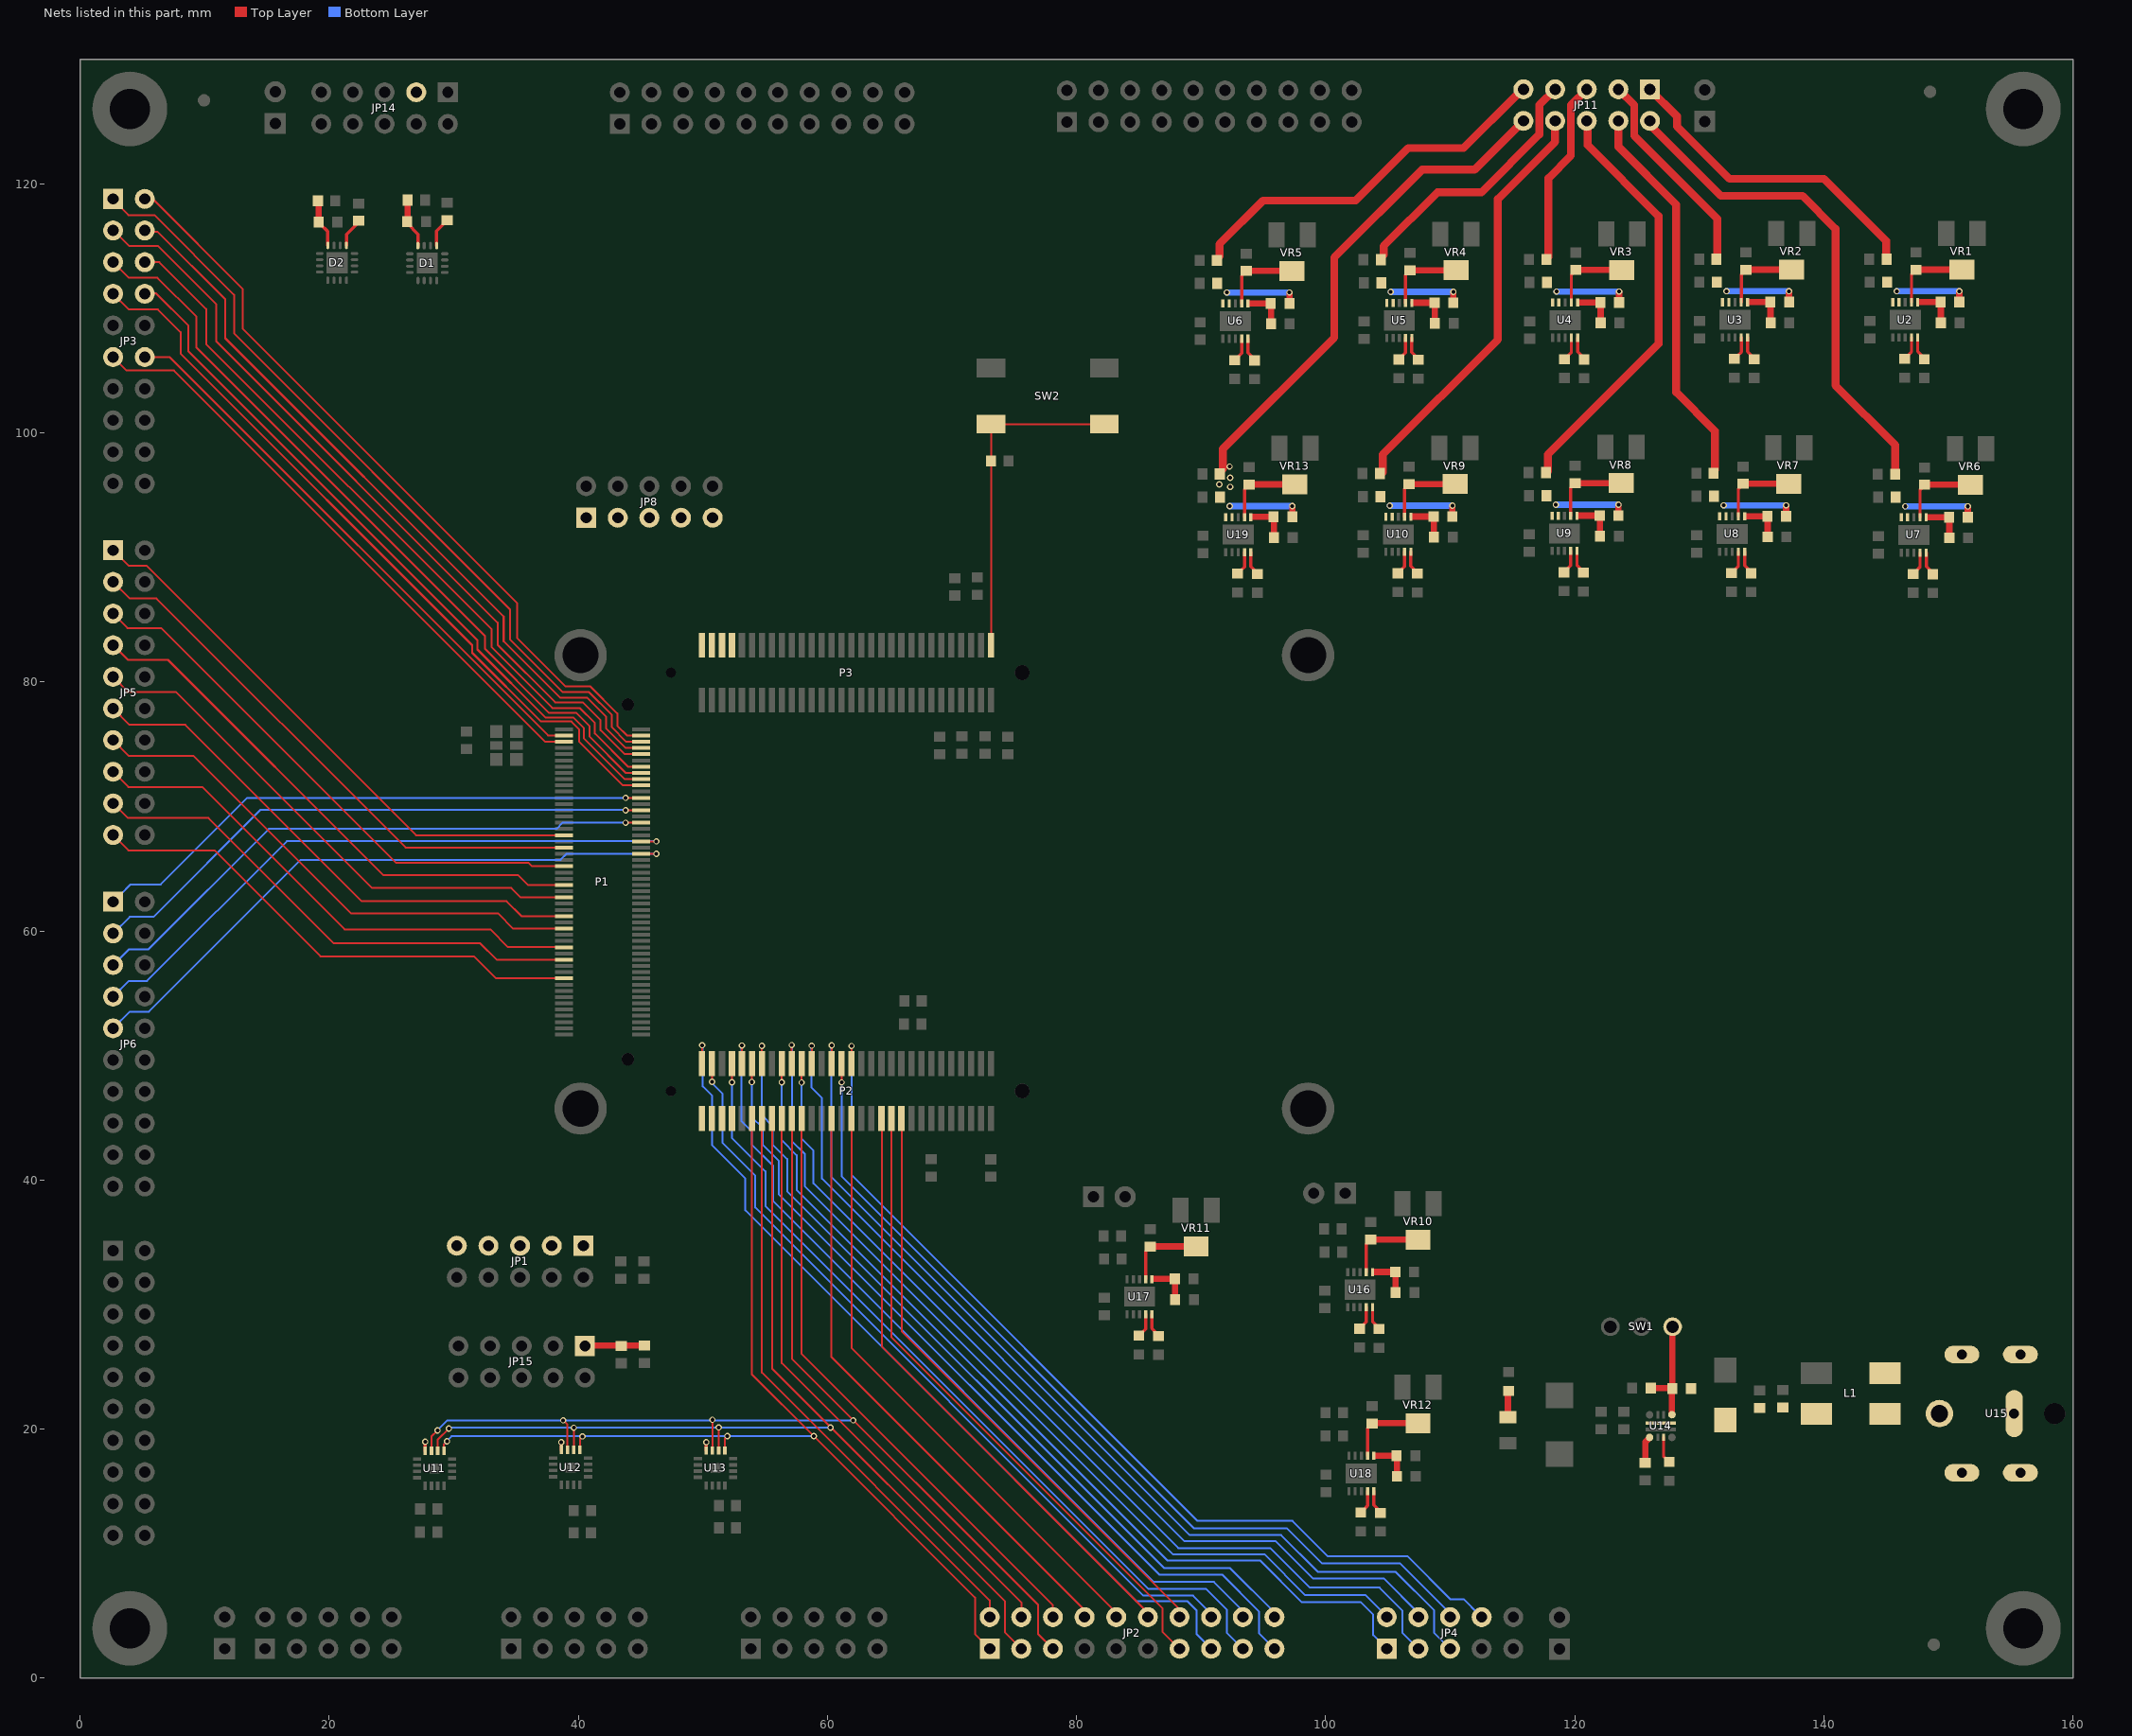
[diagram p0: the nets of this part, all layers, seen from the top]
# Altium PCB MISC82195.PcbDoc (part 5 of 8)
Units mm, origin at the board's own origin, x right, y up, seen from the top; angles counter-clockwise.
Board outline 160 x 130 mm, 4 copper layers (Top Layer, GND, POWER, Bottom Layer); 214 components, 251 nets, 1068 pads, 1218 vias.

## Via types
v1: diameter 0.508, hole 0.305, Top Layer to Bottom Layer, 1218 vias

## Nets (pads, with @x,y where several pads share a name; then routed paths per layer and width w, separated by ;. In a path a pad name is that pad's centre, name@x,y a point inside that pad or via, vN(x,y) a via of type N, cw(c..) or ccw(c..) an arc to the next point about the centre after c; other vN are vias at no path point) (continued)
LDO_1: C14.2 C15.2 JP11.1 R1.2 U2.9 U2.10 | length 31.8
  Top Layer w0.508: R1.2@150.86,110.49 v1(150.86,111.363)
  Top Layer w0.635: JP11.1@126.035,127.584 128.194,125.425 128.194,124.612 132.41,120.396 140.005,120.396 144.983,115.418 C14.2@144.983,113.995
  Bottom Layer w0.508: v1(145.838,111.363) v1(150.86,111.363)
LDO_2: C17.2 C18.2 JP11.3 R2.2 U3.9 U3.10 | length 22.5
  Top Layer w0.508: R2.2@137.194,110.49 v1(137.194,111.363)
  Top Layer w0.635: JP11.3@123.495,127.584 124.765,126.314 124.765,123.85 131.445,117.17 C17.2@131.445,114.3
  Bottom Layer w0.508: v1(132.173,111.363) v1(137.194,111.363)
LDO_3: C20.2 C21.2 JP11.5 R3.2 U4.9 U4.10 | length 20.6
  Top Layer w0.508: R3.2@123.555,110.465 v1(123.555,111.337)
  Top Layer w0.635: C20.2@117.881,114.122 117.881,120.447 119.685,122.25 119.685,126.314 JP11.5@120.955,127.584
  Bottom Layer w0.508: v1(118.533,111.337) v1(123.555,111.337)
LDO_4: C26.2 C27.2 JP11.7 R13.2 U5.9 U5.10 | length 26.9
  Top Layer w0.508: R13.2@110.245,110.439 v1(110.245,111.312)
  Top Layer w0.635: C26.2@104.648,114.3 104.648,114.986 108.966,119.304 112.497,119.304 117.145,123.952 117.145,126.314 JP11.7@118.415,127.584
  Bottom Layer w0.508: v1(105.223,111.312) v1(110.245,111.312)
LDO_5: C29.2 C30.2 JP11.9 R14.2 U6.9 U6.10 | length 36.4
  Top Layer w0.508: R14.2@97.088,110.388 v1(97.088,111.261)
  Top Layer w0.635: C29.2@91.465,114.173 91.465,115.138 94.971,118.643 102.413,118.643 106.629,122.86 111.074,122.86 JP11.9@115.443,127.229 ; JP11.9@115.494,127.178 JP11.9@115.545,127.229 ; JP11.9@115.532,127.241 JP11.9@115.875,127.584
  Bottom Layer w0.508: v1(92.066,111.261) v1(97.088,111.261)
LDO_6: C32.2 C33.2 JP11.2 R15.2 U7.9 U7.10 | length 46.2
  Top Layer w0.508: R15.2@151.545,93.218 v1(151.545,94.091)
  Top Layer w0.635: JP11.2@126.035,125.044 126.035,124.714 131.724,119.024 138.278,119.024 140.919,116.383 140.919,103.81 145.72,99.009 C32.2@145.72,96.774
  Bottom Layer w0.508: v1(146.524,94.091) v1(151.545,94.091)
LDO_7: C38.2 C39.2 JP11.4 R25.2 U8.9 U8.10 | length 37.1
  Top Layer w0.508: R25.2@136.966,93.294 v1(136.966,94.167)
  Top Layer w0.635: JP11.4@123.495,125.044 123.495,122.961 128.143,118.313 128.143,103.251 131.242,100.152 C38.2@131.242,97.028
  Bottom Layer w0.508: v1(131.944,94.167) v1(136.966,94.167)
LDO_8: C41.2 C42.2 JP11.6 R26.2 U9.9 U9.10 | length 40.1
  Top Layer w0.508: R26.2@123.504,93.345 v1(123.504,94.218)
  Top Layer w0.635: C41.2@117.831,96.901 117.831,98.247 126.721,107.137 126.721,117.399 121.031,123.088 JP11.6@121.031,124.892 ; JP11.6@120.955,124.892 JP11.6@120.955,125.044
  Bottom Layer w0.508: v1(118.482,94.218) v1(123.504,94.218)
LDO_9: C44.2 C45.2 JP11.8 R27.2 U10.9 U10.10 | length 39.8
  Top Layer w0.508: R27.2@110.169,93.269 v1(110.169,94.141)
  Top Layer w0.635: C44.2@104.572,96.825 104.572,98.247 113.817,107.493 113.817,118.77 118.415,123.368 JP11.8@118.415,125.044
  Bottom Layer w0.508: v1(105.147,94.141) v1(110.169,94.141)
LDO_10: C81.2 C82.2 JP11.10 JP14.3 R55.2 U11.16 U12.16 U13.16 U19.9 U19.10 | length 48.3
  Top Layer w0.279: U11.16@27.714,18.258 v1(27.714,18.977) ; v1(38.633,18.948) 38.636,18.946 U12.16@38.636,18.334 ; U13.16@50.269,18.283 v1(50.269,18.946)
  Top Layer w0.508: R55.2@97.316,93.243 v1(97.316,94.116)
  Top Layer w0.635: C81.2@91.745,97.104 91.745,98.704 100.686,107.645 100.686,114.071 107.747,121.133 111.963,121.133 JP11.10@115.875,125.044
  Bottom Layer w0.508: v1(92.295,94.116) v1(97.316,94.116)
  other v1: 92.329,95.656 91.465,95.86 92.329,96.393 92.278,97.282
M_RESET_IN_N: C8.1 P3.C59 SW2.3 SW2.4 | length 26.4
  Top Layer w0.152: SW2.3@73.123,100.696 SW2.4@81.9,100.696 ; P3.C59@73.137,82.939 73.137,99.212 SW2.3@73.137,100.573
NetC22_2: C22.2 U2.7 VR1.2 | length 6.4
  Top Layer w0.254: U2.7@147.025,110.479 147.025,112.71 C22.2@147.295,112.979
  Top Layer w0.508: C22.2@147.292,113.104 VR1.2@151.071,113.104
NetC23_2: C23.2 U3.7 VR2.2 | length 6.4
  Top Layer w0.254: U3.7@133.36,110.479 133.36,112.71 C23.2@133.629,112.979
  Top Layer w0.508: C23.2@133.627,113.104 VR2.2@137.406,113.104
NetC24_2: C24.2 U4.7 VR3.2 | length 6.4
  Top Layer w0.254: U4.7@119.72,110.454 119.72,112.684 C24.2@119.99,112.954
  Top Layer w0.508: C24.2@119.987,113.079 VR3.2@123.766,113.079
NetC34_2: C34.2 U5.7 VR4.2 | length 6.4
  Top Layer w0.254: U5.7@106.41,110.428 106.41,112.659 C34.2@106.68,112.928
  Top Layer w0.508: C34.2@106.678,113.053 VR4.2@110.457,113.053
NetC35_2: C35.2 U6.7 VR5.2 | length 6.4
  Top Layer w0.254: U6.7@93.253,110.377 93.253,112.608 C35.2@93.523,112.878
  Top Layer w0.508: C35.2@93.521,113.002 VR5.2@97.3,113.002
NetC36_2: C36.2 U7.7 VR6.2 | length 6.4
  Top Layer w0.254: U7.7@147.711,93.207 147.711,95.438 C36.2@147.98,95.707
  Top Layer w0.508: C36.2@147.978,95.832 VR6.2@151.757,95.832
NetC46_2: C46.2 U8.7 VR7.2 | length 6.4
  Top Layer w0.254: U8.7@133.131,93.283 133.131,95.514 C46.2@133.401,95.783
  Top Layer w0.508: C46.2@133.399,95.908 VR7.2@137.178,95.908
NetC47_2: C47.2 U9.7 VR8.2 | length 6.4
  Top Layer w0.254: U9.7@119.669,93.334 119.669,95.565 C47.2@119.939,95.834
  Top Layer w0.508: C47.2@119.937,95.959 VR8.2@123.716,95.959
NetC48_2: C48.2 U10.7 VR9.2 | length 6.4
  Top Layer w0.254: U10.7@106.334,93.258 106.334,95.488 C48.2@106.604,95.758
  Top Layer w0.508: C48.2@106.602,95.883 VR9.2@110.381,95.883
NetC57_2: C57.2 D1.16 R37.1 | length 4
  Top Layer w0.254: R37.1@26.289,117.016 26.289,116.789 27.13,115.948 D1.16@27.13,115.024
  Top Layer w0.508: R37.1@26.291,117.016 C57.2@26.291,118.679
NetC58_1: C58.1 D1.13 | length 2.1
  Top Layer w0.254: D1.13@28.63,115.024 28.63,116.209 C58.1@29.286,116.865
NetC59_2: C59.2 D2.16 R38.1 | length 3.6
  Top Layer w0.254: R38.1@19.329,116.738 19.891,116.177 D2.16@19.891,115.05
  Top Layer w0.508: R38.1@19.151,116.926 C59.2@19.151,118.592
NetC60_1: C60.1 D2.13 | length 2.2
  Top Layer w0.254: D2.13@21.391,115.05 21.391,115.93 C60.1@22.301,116.84
NetC61_2: C61.2 C62.2 JP15.1 | length 4.6
  Top Layer w0.508: JP15.1@40.752,26.711 C62.2@45.323,26.711
NetC65_2: C65.2 C66.2 D4.2 L1.4 R41.1 U14.5
NetC67_2: C67.2 U14.7 | length 2.2
  Top Layer w0.508: C67.2@125.774,17.406 C67.2@125.654,17.286 125.654,18.948 U14.7@125.882,19.177
NetC77_2: C77.2 U16.7 VR10.2 | length 6.9
  Top Layer w0.254: U16.7@103.261,32.603 103.261,34.833 C77.2@103.53,35.103
  Top Layer w0.508: C77.2@103.528,35.228 107.417,35.228 107.698,35.228 VR10.2@107.747,35.179
NetC78_2: C78.2 U17.7 VR11.2 | length 6.4
  Top Layer w0.254: U17.7@85.557,32.044 85.557,34.274 C78.2@85.827,34.544
  Top Layer w0.508: C78.2@85.824,34.669 VR11.2@89.603,34.669
NetC79_2: C79.2 U18.7 VR12.2 | length 6.4
  Top Layer w0.254: U18.7@103.362,17.845 103.362,20.076 C79.2@103.632,20.345
  Top Layer w0.508: C79.2@103.63,20.47 VR12.2@107.409,20.47
NetC83_2: C83.2 U19.7 VR13.2 | length 6.4
  Top Layer w0.254: U19.7@93.482,93.232 93.482,95.463 C83.2@93.751,95.733
  Top Layer w0.508: C83.2@93.749,95.857 VR13.2@97.528,95.857
NetJP1_1: JP1.1 JP1.3 JP1.5 JP1.7 JP1.9 P2.A2 P2.A4 P2.A6 P2.A8
NetJP8_1: JP8.1 JP8.3 JP8.5 JP8.7 JP8.9 P3.C1 P3.C3 P3.C5 P3.C7
NetL1_1: L1.1 U15.1
NetL1_2: L1.2 U15.2 U15.3
NetLED1_2: LED1.2 R42.2 | length 1.9
  Top Layer w0.508: LED1.2@114.63,20.964 R42.2@114.63,22.835
NetR1_1: R1.1 R7.2 U2.6 | length 3.4
  Top Layer w0.508: 147.676,110.491 149.378,110.491 R7.2@149.378,108.839
NetR2_1: R2.1 R8.2 U3.6 | length 3.4
  Top Layer w0.508: 134.011,110.491 135.713,110.491 R8.2@135.713,108.839
NetR3_1: R3.1 R9.2 U4.6 | length 3.4
  Top Layer w0.508: 120.371,110.465 122.073,110.465 R9.2@122.073,108.814
NetR4_1: R4.1 U2.4 | length 1.6
  Top Layer w0.254: R4.1@146.71,106.172 147.025,106.487 U2.4@147.025,107.656
NetR5_1: R5.1 U3.4 | length 1.6
  Top Layer w0.254: R5.1@133.045,106.172 133.36,106.487 U3.4@133.36,107.656
NetR6_1: R6.1 U4.4 | length 1.6
  Top Layer w0.254: R6.1@119.405,106.147 119.72,106.461 U4.4@119.72,107.631
NetR10_2: R10.2 U2.5 | length 1.7
  Top Layer w0.254: U2.5@147.525,107.656 147.525,106.526 R10.2@147.904,106.147
NetR11_2: R11.2 U3.5 | length 1.7
  Top Layer w0.254: U3.5@133.86,107.656 133.86,106.526 R11.2@134.239,106.147
NetR12_2: R12.2 U4.5 | length 1.7
  Top Layer w0.254: U4.5@120.22,107.631 120.22,106.501 R12.2@120.599,106.121
NetR13_1: R13.1 R19.2 U5.6 | length 3.4
  Top Layer w0.508: 107.062,110.44 108.764,110.44 R19.2@108.764,108.788
NetR14_1: R14.1 R20.2 U6.6 | length 3.4
  Top Layer w0.508: 93.905,110.389 95.606,110.389 R20.2@95.606,108.737
NetR15_1: R15.1 R21.2 U7.6 | length 3.4
  Top Layer w0.508: 148.362,93.219 150.064,93.219 R21.2@150.064,91.567
NetR16_1: R16.1 U5.4 | length 1.6
  Top Layer w0.254: R16.1@106.096,106.121 106.41,106.436 U5.4@106.41,107.605
NetR17_1: R17.1 U6.4 | length 1.6
  Top Layer w0.254: R17.1@92.939,106.07 93.253,106.385 U6.4@93.253,107.555
NetR18_1: R18.1 U7.4 | length 1.6
  Top Layer w0.254: R18.1@147.396,88.9 147.711,89.215 U7.4@147.711,90.384
NetR22_2: R22.2 U5.5 | length 1.7
  Top Layer w0.254: U5.5@106.91,107.605 106.91,106.475 R22.2@107.29,106.096
NetR23_2: R23.2 U6.5 | length 1.7
  Top Layer w0.254: U6.5@93.753,107.555 93.753,106.424 R23.2@94.132,106.045
NetR24_2: R24.2 U7.5 | length 1.7
  Top Layer w0.254: U7.5@148.211,90.384 148.211,89.254 R24.2@148.59,88.875
NetR25_1: R25.1 R31.2 U8.6 | length 3.4
  Top Layer w0.508: 133.783,93.295 135.484,93.295 R31.2@135.484,91.643
NetR26_1: R26.1 R32.2 U9.6 | length 3.4
  Top Layer w0.508: 120.321,93.346 122.022,93.346 R32.2@122.022,91.694
NetR27_1: R27.1 R33.2 U10.6 | length 3.4
  Top Layer w0.508: 106.986,93.27 108.687,93.27 R33.2@108.687,91.618
NetR28_1: R28.1 U8.4 | length 1.6
  Top Layer w0.254: R28.1@132.817,88.976 133.131,89.291 U8.4@133.131,90.46
NetR29_1: R29.1 U9.4 | length 1.6
  Top Layer w0.254: R29.1@119.355,89.027 119.669,89.342 U9.4@119.669,90.511
NetR30_1: R30.1 U10.4 | length 1.6
  Top Layer w0.254: R30.1@106.02,88.951 106.334,89.265 U10.4@106.334,90.435
NetR34_2: R34.2 U8.5 | length 1.7
  Top Layer w0.254: U8.5@133.631,90.46 133.631,89.33 R34.2@134.01,88.951
NetR35_2: R35.2 U9.5 | length 1.7
  Top Layer w0.254: U9.5@120.169,90.511 120.169,89.381 R35.2@120.548,89.002
NetR36_2: R36.2 U10.5 | length 1.7
  Top Layer w0.254: U10.5@106.834,90.435 106.834,89.305 R36.2@107.213,88.925
NetR39_1: R39.1 R41.2 SW1.3 U14.1 | length 8.7
  Top Layer w0.508: R39.1@126.213,23.292 127.787,23.292 127.798,23.281 U14.1@127.798,21.159 ; R41.2@127.821,23.266 SW1.3@127.821,28.253
NetR40_1: R40.1 U14.9 | length 1.9
  Top Layer w0.254: U14.9@127.123,19.339 127.123,17.834 R40.1@127.381,17.577
NetR43_1: R43.1 R49.2 U16.6 | length 3.4
  Top Layer w0.508: 103.912,32.614 105.614,32.614 R49.2@105.614,30.963
NetR44_1: R44.1 R50.2 U17.6 | length 3.4
  Top Layer w0.508: 86.208,32.056 87.91,32.056 R50.2@87.91,30.404
NetR45_1: R45.1 R51.2 U18.6 | length 3.4
  Top Layer w0.508: 104.014,17.857 105.716,17.857 R51.2@105.716,16.205
NetR46_1: R46.1 U16.4 | length 1.6
  Top Layer w0.254: R46.1@102.946,28.296 103.261,28.61 U16.4@103.261,29.78
NetR47_1: R47.1 U17.4 | length 1.6
  Top Layer w0.254: R47.1@85.242,27.737 85.557,28.051 U17.4@85.557,29.221
NetR48_1: R48.1 U18.4 | length 1.6
  Top Layer w0.254: R48.1@103.048,13.538 103.362,13.853 U18.4@103.362,15.022
NetR52_2: R52.2 U16.5 | length 1.7
  Top Layer w0.254: U16.5@103.761,29.78 103.761,28.65 R52.2@104.14,28.27
NetR53_2: R53.2 U17.5 | length 1.7
  Top Layer w0.254: U17.5@86.057,29.221 86.057,28.091 R53.2@86.436,27.711
NetR54_2: R54.2 U18.5 | length 1.7
  Top Layer w0.254: U18.5@103.862,15.022 103.862,13.892 R54.2@104.242,13.513
NetR55_1: R55.1 R57.2 U19.6 | length 3.4
  Top Layer w0.508: 94.133,93.244 95.835,93.244 R57.2@95.835,91.592
NetR56_1: R56.1 U19.4 | length 1.6
  Top Layer w0.254: R56.1@93.167,88.925 93.482,89.24 U19.4@93.482,90.41
NetR58_2: R58.2 U19.5 | length 1.7
  Top Layer w0.254: U19.5@93.982,90.41 93.982,89.279 R58.2@94.361,88.9
PW1: JP2.1 P2.A12 U11.13 U12.13 U13.13 | length 83.7
  Top Layer w0.152: U11.13@29.214,18.258 29.214,18.775 v1(29.464,19.025) ; U12.13@40.136,18.334 40.136,19.207 v1(40.335,19.406) ; U13.13@51.769,18.521 U13.13@51.769,18.283 51.769,19.232 v1(51.968,19.431) ; P2.A12@53.937,44.938 53.924,44.925 53.924,24.409 v1@58.877,19.456 ; v1(58.903,19.431) v1@58.877,19.456 ; JP2.1@73.025,2.362 71.857,3.531 71.857,6.477 v1@58.877,19.456
  Bottom Layer w0.152: v1@29.515,19.126 29.82,19.431 30.353,19.431 ; 30.15,19.431 30.353,19.431 ; v1@58.877,19.431 v1(51.968,19.431) 30.353,19.431
PW2: JP2.3 P2.A16 U11.14 U12.14 U13.14 | length 87.3
  Top Layer w0.152: U11.14@28.714,18.258 28.714,19.138 v1(29.616,20.041) ; U12.14@39.636,18.334 v1(39.636,20.105) ; U13.14@51.269,18.283 v1(51.269,20.129) ; P2.A16@55.55,44.926 55.55,24.867 74.27,6.147 74.27,3.658 JP2.3@75.565,2.362
  Bottom Layer w0.152: v1@29.667,20.117 60.274,20.117 v1(60.249,20.117)
PW3: JP2.5 P2.A20 U11.15 U12.15 U13.15 | length 91.6
  Top Layer w0.152: U11.15@28.214,18.258 28.214,19.4 v1(28.702,19.888) ; v1(38.786,20.701) 39.136,20.351 U12.15@39.136,18.334 ; U13.15@50.769,18.283 v1(50.769,20.747) ; P2.A20@57.15,44.926 57.15,25.654 76.911,5.893 76.911,3.556 JP2.5@78.105,2.362
  Bottom Layer w0.152: v1@28.804,20.015 29.489,20.701 v1(38.786,20.701) v1(62.078,20.701)
PW7: JP2.13 P2.A40 | length 52.1
  Top Layer w0.152: P2.A40@65.151,44.925 65.151,27.356 86.919,5.588 86.919,3.708 JP2.13@88.265,2.362
PW8: JP2.15 P2.A1 | length 69.5
  Top Layer w0.152: P2.A1@49.937,49.338 v1(49.937,50.824)
  Bottom Layer w0.152: v1@49.987,50.749 49.987,47.523 50.724,46.787 50.724,46.38 ; 50.724,46.685 50.724,46.38 ; JP2.15@90.805,2.362 89.637,3.531 89.637,5.436 88.875,6.198 84.785,6.198 53.416,37.567 53.416,40.107 50.724,42.799 50.724,46.38
PW9: JP2.17 P2.A7 | length 66.7
  Top Layer w0.152: v1(52.337,47.842) P2.A7@52.337,49.338
  Bottom Layer w0.152: v1@52.451,47.828 52.324,47.701 52.324,43.383 55.016,40.691 55.016,37.922 85.776,7.163 90.399,7.163 92.075,5.486 92.075,3.632 JP2.17@93.345,2.362
PW10: JP2.19 P2.A11 | length 67.3
  Top Layer w0.152: v1(53.937,47.866) P2.A11@53.937,49.338
  Bottom Layer w0.152: v1@53.924,47.828 53.924,45.06 54.813,44.171 54.813,42.824 56.109,41.529 56.109,38.837 86.639,8.306 91.694,8.306 94.64,5.359 94.64,3.607 JP2.19@95.885,2.362
PW11: JP4.1 P2.A17 | length 74.3
  Top Layer w0.152: v1(56.337,47.854) P2.A17@56.337,49.338
  Bottom Layer w0.152: v1@56.337,47.955 56.337,43.18 57.531,41.986 57.531,39.218 87.3,9.449 94.742,9.449 98.095,6.096 102.819,6.096 103.81,5.105 103.81,3.454 JP4.1@104.902,2.362
PW12: JP4.3 P2.A21 | length 75.1
  Top Layer w0.152: v1(57.937,47.828) P2.A21@57.937,49.338
  Bottom Layer w0.152: v1@58.014,47.854 57.937,47.777 57.937,43.307 58.877,42.367 58.877,39.726 88.163,10.439 95.555,10.439 98.73,7.264 104.318,7.264 106.172,5.41 106.172,3.632 JP4.3@107.442,2.362
PW13: JP4.5 P2.A27 | length 78.4
  Top Layer w0.152: P2.A27@60.337,49.338 v1(60.337,50.812)
  Bottom Layer w0.152: v1@60.325,50.724 60.325,40.234 89.078,11.481 96.418,11.481 99.365,8.534 105.613,8.534 108.712,5.436 108.712,3.632 JP4.5@109.982,2.362
PW14: JP4.8 P2.A31 | length 77
  Top Layer w0.152: P2.A31@61.937,49.338 v1(61.937,50.761)
  Bottom Layer w0.152: v1@61.951,50.673 61.951,40.386 89.713,12.624 97.333,12.624 100.178,9.779 106.578,9.779 110.033,6.325 111.1,6.325 112.268,5.156 JP4.8@112.522,4.902
PW15: JP4.6 P2.A29 | length 72.8
  Top Layer w0.152: v1(61.137,47.829) P2.A29@61.137,49.338
  Bottom Layer w0.152: v1@61.29,47.854 61.138,47.701 61.138,40.31 89.408,12.04 96.876,12.04 99.708,9.207 105.981,9.207 109.982,5.207 JP4.6@109.982,4.902
PW16: JP4.4 P2.A23 | length 75.1
  Top Layer w0.152: P2.A23@58.737,49.338 v1(58.737,50.787)
  Bottom Layer w0.152: v1@58.725,50.775 58.725,47.422 59.563,46.584 59.563,40.107 88.671,10.998 95.987,10.998 98.996,7.988 104.686,7.988 107.442,5.232 JP4.4@107.442,4.902
PW17: JP4.2 P2.A19 | length 74.4
  Top Layer w0.152: P2.A19@57.137,49.338 v1(57.137,50.838)
  Bottom Layer w0.152: v1@57.137,50.749 v1(57.137,50.838) ; v1@57.15,50.749 57.15,43.129 58.204,42.075 58.204,39.484 87.732,9.957 95.072,9.957 98.361,6.667 103.213,6.667 104.902,4.978 JP4.2@104.902,4.902
PW18: JP2.20 P2.A13 | length 67.5
  Top Layer w0.152: P2.A13@54.737,49.338 v1(54.737,50.774)
  Bottom Layer w0.152: v1(54.737,50.774) 54.737,45.212 55.601,44.348 55.601,42.85 56.769,41.681 56.769,39.091 87.02,8.839 92.329,8.839 95.885,5.283 JP2.20@95.885,4.902
PW19: JP2.18 P2.A9 | length 66.8
  Top Layer w0.152: P2.A9@53.137,49.338 v1(53.137,50.799)
  Bottom Layer w0.152: v1@53.111,50.724 53.111,44.729 53.924,43.917 53.924,42.85 55.651,41.123 55.651,38.278 86.208,7.722 91.034,7.722 93.345,5.41 JP2.18@93.345,4.902
PW20: JP2.16 P2.A3 | length 63.2
  Top Layer w0.152: v1(50.737,47.891) P2.A3@50.737,49.338
  Bottom Layer w0.152: v1@50.749,47.752 51.562,46.939 51.562,43.002 54.204,40.361 54.204,37.795 85.369,6.629 89.357,6.629 90.805,5.182 JP2.16@90.805,4.902
PW21: JP2.14 P2.A42 | length 49.5
  Top Layer w0.152: P2.A42@65.937,44.938 65.964,44.912 65.964,43.409 ; 65.964,43.637 65.964,43.409 ; JP2.14@88.265,4.902 88.265,5.563 65.964,27.864 65.964,43.409
PW22: JP2.12 P2.A38 | length 48.9
  Top Layer w0.152: P2.A38@64.337,44.938 64.364,44.912 64.364,26.619 85.725,5.258 JP2.12@85.725,4.902
PW23: JP2.10 P2.A32 | length 48.8
  Top Layer w0.152: P2.A32@61.951,44.925 61.951,26.492 83.185,5.258 JP2.10@83.185,4.902
PW24: JP2.8 P2.A28 | length 48.5
  Top Layer w0.152: P2.A28@60.337,44.938 60.325,44.926 60.325,25.781 80.645,5.461 JP2.8@80.645,4.902
PW25: JP2.6 P2.A22 | length 48.4
  Top Layer w0.152: P2.A22@57.937,44.938 57.937,26.035 78.105,5.867 JP2.6@78.105,4.902
PW26: JP2.4 P2.A18 | length 48
  Top Layer w0.152: P2.A18@56.337,44.938 56.337,25.298 75.565,6.071 JP2.4@75.565,4.902
PW27: JP2.2 P2.A14 | length 47.6
  Top Layer w0.152: P2.A14@54.737,44.938 54.737,24.536 73.025,6.248 JP2.2@73.025,4.902
PW28: JP3.1 P1.B5 | length 64.3
  Top Layer w0.152: JP3.1@2.658,118.781 JP3.1@3.239,118.199 ; JP3.1@3.2,118.161 3.886,117.475 5.969,117.475 12.37,111.074 12.37,107.975 34.519,85.827 34.519,83.414 38.76,79.172 40.869,79.172 42.672,77.368 42.672,76.378 43.861,75.188 P1.B5@45.038,75.188
PW29: JP3.2 P1.B3 | length 61.8
  Top Layer w0.152: JP3.2@5.198,118.781 JP3.2@5.334,118.781 ; JP3.2@5.334,118.72 5.893,118.72 13.056,111.557 13.056,108.356 35.077,86.335 35.077,83.541 38.964,79.654 40.945,79.654 43.129,77.47 43.129,76.479 43.92,75.688 P1.B3@45.038,75.688
PW30: JP3.3 P1.B9 | length 63
  Top Layer w0.152: JP3.3@2.658,116.241 JP3.3@2.998,115.901 ; JP3.3@3.023,115.926 3.962,114.986 6.274,114.986 10.922,110.338 10.922,107.366 33.528,84.76 33.528,82.982 38.151,78.359 40.361,78.359 41.783,76.937 41.783,76.124 43.718,74.188 P1.B9@45.038,74.188
PW31: JP3.4 P1.B7 | length 60.6
  Top Layer w0.152: JP3.4@5.198,116.241 JP3.4@5.41,116.241 ; JP3.4@5.41,116.154 6.223,116.154 11.659,110.719 11.659,107.594 34.011,85.242 34.011,83.261 38.532,78.74 40.691,78.74 42.24,77.191 42.24,76.251 43.803,74.688 P1.B7@45.038,74.688
PW32: JP3.5 P1.B15 | length 61.9
  Top Layer w0.152: JP3.5@2.658,113.701 3.913,112.446 6.223,112.446 9.347,109.322 9.347,106.832 32.512,83.668 32.512,82.652 37.668,77.495 39.853,77.495 40.894,76.454 40.894,75.616 43.821,72.688 P1.B15@45.038,72.688
PW33: JP3.6 P1.B13 | length 59.6
  Top Layer w0.152: JP3.6@5.198,113.701 JP3.6@5.588,113.701 ; JP3.6@5.588,113.69 6.375,113.69 10.135,109.931 10.135,107.112 33.045,84.201 33.045,82.779 37.922,77.902 40.107,77.902 41.326,76.683 41.326,75.844 43.982,73.188 P1.B13@45.038,73.188
PW34: JP3.7 P1.B19 | length 60.7
  Top Layer w0.152: JP3.7@2.658,111.161 3.913,109.906 6.248,109.906 8.077,108.077 8.077,106.35 31.483,82.944 31.483,82.334 37.008,76.81 39.446,76.81 40.056,76.2 40.056,75.209 43.577,71.688 P1.B19@45.038,71.688
PW35: JP3.8 P1.B17 | length 58.1
  Top Layer w0.152: JP3.8@5.198,111.161 JP3.8@5.334,111.161 ; JP3.8@5.334,111.201 6.096,111.201 8.712,108.585 8.712,106.528 31.902,83.337 31.902,82.601 37.389,77.114 39.624,77.114 40.437,76.302 40.437,75.489 43.737,72.188 P1.B17@45.038,72.188
PW36: JP3.11 P1.B6 | length 49
  Top Layer w0.152: JP3.11@2.658,106.081 3.735,105.004 7.544,105.004 37.359,75.188 P1.B6@38.866,75.188
PW37: JP3.12 P1.B4 | length 46.3
  Top Layer w0.152: JP3.12@5.198,106.081 7.178,106.081 37.567,75.692 37.57,75.688 P1.B4@38.866,75.688
PW38: JP5.1 P1.B36 | length 46.3
  Top Layer w0.152: JP5.1@2.658,90.561 3.913,89.306 5.367,89.306 26.983,67.691 37.287,67.691 ; 37.914,67.691 37.287,67.691 ; P1.B36@38.862,67.691 37.287,67.691
PW39: JP5.3 P1.B40 | length 45.3
  Top Layer w0.152: JP5.3@2.658,88.021 3.989,86.69 6.147,86.69 26.137,66.7 37.262,66.7 ; 37.821,66.7 37.262,66.7 ; P1.B40@38.583,66.7 37.262,66.7
PW40: JP5.5 P1.B46 | length 44.6
  Top Layer w0.152: JP5.5@2.658,85.481 3.811,84.328 6.528,84.328 25.4,65.456 36.017,65.456 36.285,65.188 P1.B46@38.866,65.188
PW41: JP5.7 P1.B52 | length 44.2
  Top Layer w0.152: JP5.7@2.658,82.941 3.836,81.763 7.061,81.763 24.333,64.491 35.154,64.491 35.956,63.688 P1.B52@38.866,63.688
PW42: JP5.9 P1.B56 | length 43.5
  Top Layer w0.152: JP5.9@2.658,80.401 3.887,79.172 7.722,79.172 23.444,63.449 34.62,63.449 35.381,62.688 P1.B56@38.866,62.688
PW43: JP5.11 P1.B62 | length 43.1
  Top Layer w0.152: JP5.11@2.658,77.861 3.963,76.556 8.458,76.556 22.631,62.382 34.239,62.382 35.433,61.188 P1.B62@38.866,61.188
PW44: JP5.13 P1.B66 | length 42.5
  Top Layer w0.152: JP5.13@2.658,75.321 3.938,74.041 9.119,74.041 21.768,61.392 33.579,61.392 34.782,60.188 P1.B66@38.866,60.188
PW45: JP5.15 P1.B72 | length 41.8
  Top Layer w0.152: JP5.15@2.658,72.781 3.887,71.552 9.804,71.552 21.234,60.122 32.944,60.122 34.366,58.699 P1.B72@38.583,58.699
PW46: JP5.17 P1.B76 | length 41.4
  Top Layer w0.152: JP5.17@2.658,70.241 3.836,69.063 10.312,69.063 20.371,59.004 32.131,59.004 33.447,57.688 P1.B76@38.866,57.688
PW47: JP5.19 P1.B82 | length 41
  Top Layer w0.152: JP5.19@2.658,67.701 3.887,66.472 10.795,66.472 19.304,57.963 31.623,57.963 33.397,56.188 P1.B82@38.866,56.188
PW48: JP6.1 P1.B23 | length 45.9
  Top Layer w0.152: v1(43.803,70.688) P1.B23@45.038,70.688
  Bottom Layer w0.152: JP6.1@2.658,62.342 JP6.1@3.241,62.926 ; JP6.1@3.251,62.916 4.064,63.729 6.477,63.729 13.437,70.688 v1@43.891,70.688
PW49: JP6.3 P1.B27 | length 46.5
  Top Layer w0.152: v1(43.803,69.688) P1.B27@45.038,69.688
  Bottom Layer w0.152: JP6.3@2.658,59.802 3.994,61.138 5.893,61.138 14.478,69.723 v1@43.84,69.723
PW50: JP6.5 P1.B31 | length 47.1
  Top Layer w0.152: v1(43.803,68.688) P1.B31@45.038,68.688
  Bottom Layer w0.152: JP6.5@2.658,57.262 3.918,58.522 5.486,58.522 15.164,68.199 38.252,68.199 38.735,68.682 v1@43.815,68.682
PW51: JP6.7 P1.B37 | length 50
  Top Layer w0.152: P1.B37@45.038,67.188 v1(46.274,67.188)
  Bottom Layer w0.152: JP6.7@2.658,54.722 3.918,55.982 5.372,55.982 16.599,67.208 46.254,67.208 v1(46.274,67.188)
PW52: JP6.9 P1.B41 | length 51
  Top Layer w0.152: P1.B41@45.038,66.188 v1(46.274,66.188)
  Bottom Layer w0.152: JP6.9@2.658,52.182 3.994,53.518 5.537,53.518 17.725,65.706 38.579,65.706 39.065,66.192 43.739,66.192 ; 44.12,66.192 43.739,66.192 ; v1@46.27,66.192 43.739,66.192